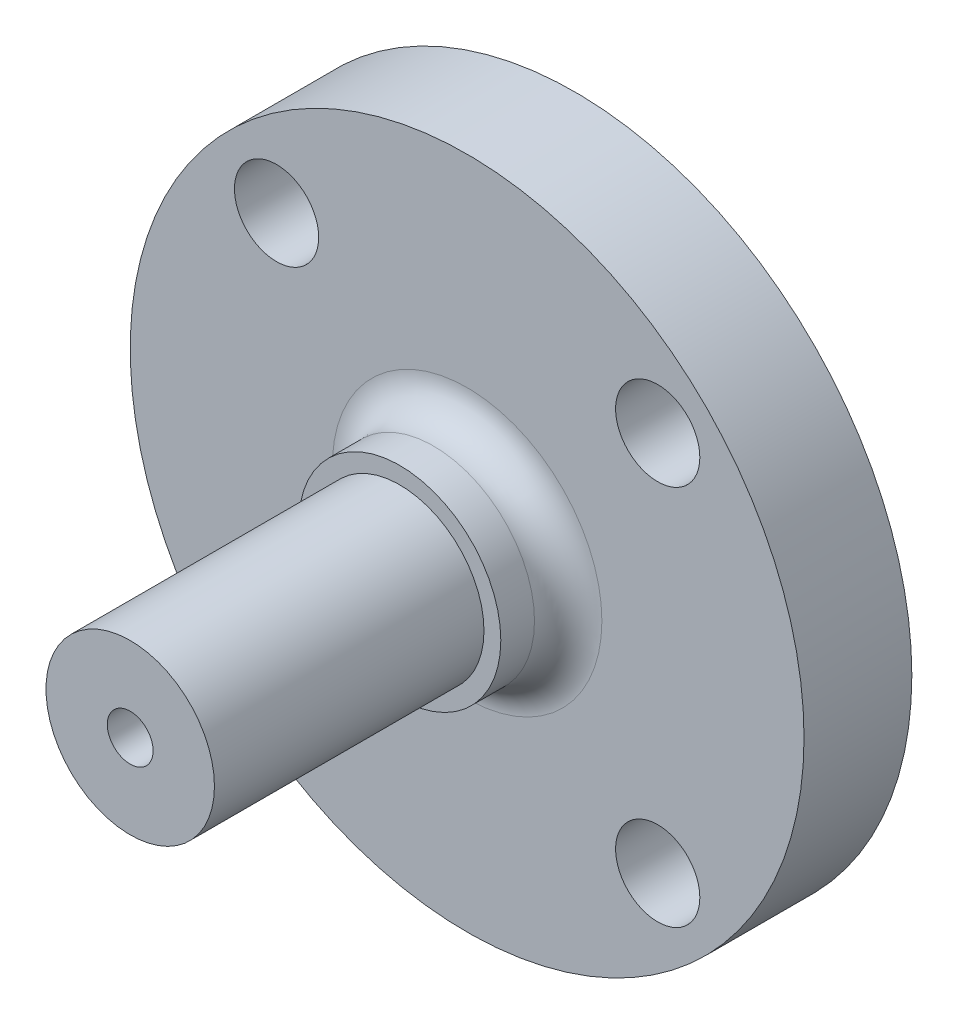
from build123d import *

# Parameters (mm, degrees)
SKETCH_1_R                = 50
EXTRUDE_1_DEPTH           = 16
SKETCH_2_R                = 15
EXTRUDE_2_DEPTH           = 10
SKETCH_3_R                = 12.5
EXTRUDE_3_DEPTH           = 40
HOLE_WIZARD_12_5_12_5_1_D = 12.5
PATTERN_CIRCULAR_1_COUNT  = 4
HOLE_WIZARD_M8_1_D        = 6.8
HOLE_WIZARD_M8_1_DEPTH    = 19.75
HOLE_WIZARD_M8_1_TIP      = 2.042926105
FILLET_1_R                = 5


with BuildPart() as part:
    # 草图1 → 凸台-拉伸1 (new body)
    with BuildSketch(Plane.XY):
        Circle(SKETCH_1_R)
    extrude(amount=EXTRUDE_1_DEPTH)

    # 草图2 → 凸台-拉伸2 (add)
    with BuildSketch(Plane.XY.offset(16)):
        Circle(SKETCH_2_R)
    extrude(amount=EXTRUDE_2_DEPTH)

    # 草图3 → 凸台-拉伸3 (add)
    with BuildSketch(Plane.XY.offset(26)):
        Circle(SKETCH_3_R)
    extrude(amount=EXTRUDE_3_DEPTH)

    # Ø12.5 (12.5) 直径孔1 (through all)
    with Locations(Plane.XY.offset(16)):
        with Locations((-28.284271247, 28.284271247)):
            hole_wizard_12_5_12_5_1 = Hole(HOLE_WIZARD_12_5_12_5_1_D / 2)

    # 阵列(圆周)1: Ø12.5 (12.5) 直径孔1 ×4 about axis
    pattern_circular_1_axis = Axis((0, 0, 0), (0, 0, 1))
    for i in range(1, PATTERN_CIRCULAR_1_COUNT):
        add(hole_wizard_12_5_12_5_1.rotate(pattern_circular_1_axis, i * 360 / PATTERN_CIRCULAR_1_COUNT), mode=Mode.SUBTRACT)

    # M8 螺纹孔1
    with Locations(Plane.XY.offset(66)):
        with Locations((0, 0)):
            Hole(HOLE_WIZARD_M8_1_D / 2, depth=HOLE_WIZARD_M8_1_DEPTH)
            with Locations((0, 0, -(HOLE_WIZARD_M8_1_DEPTH + HOLE_WIZARD_M8_1_TIP / 2))):  # 118° drill point
                Cone(0, HOLE_WIZARD_M8_1_D / 2, HOLE_WIZARD_M8_1_TIP, mode=Mode.SUBTRACT)

    # 圆角1
    fillet_1_edges = [part.edges().sort_by_distance(p)[0] for p in [
        (-15, 0, 16),
    ]]
    fillet(fillet_1_edges, radius=FILLET_1_R)


solid = part.part
